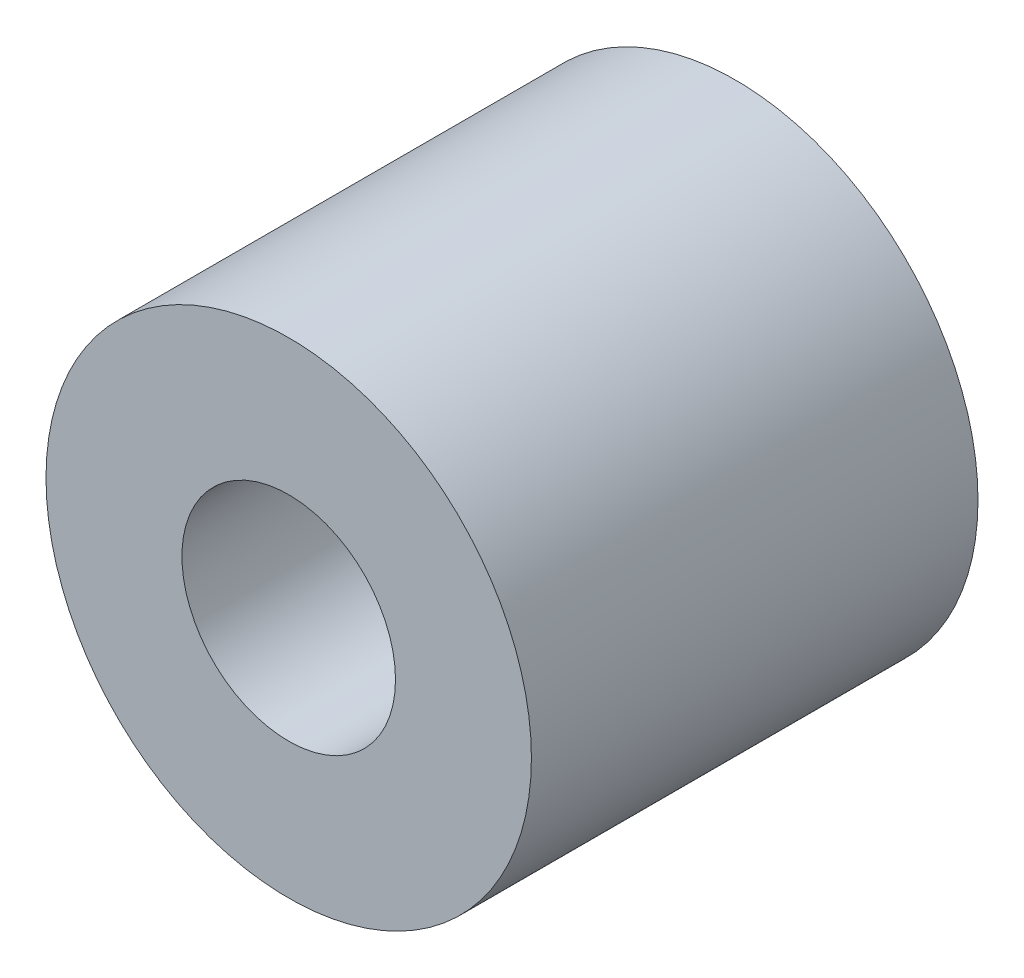
SolidWorks part; units mm, degrees
ref_plane "前视基准面" through (0, 0, 0) normal (0, 0, 1) x (1, 0, 0)
ref_plane "上视基准面" through (0, 0, 0) normal (0, 1, 0) x (1, 0, 0)
ref_plane "右视基准面" through (0, 0, 0) normal (1, 0, 0) x (0, 0, -1)
sketch "草图1" plane through (0, 0, 0) normal (0, 0, 1) x (1, 0, 0)
  circle A0 centre (0, 0) radius 12.5
  dimension "D1" = 25
extrude "凸台-拉伸1" add sketch "草图1" along normal blind 23
sketch "草图4" plane through (0, 0, 23) normal (0, 0, 1) x (1, 0, 0)
  point P0 (0, 0)
hole_wizard "M6 六角圆柱头螺钉的柱形沉头孔1" positions "草图4" profile "草图3" counterbore size "M6" standard "GB" end condition through all
sketch "草图3" plane through (0, 0, 23) normal (1, 0, 0) x (0, -1, 0)
  line L0 (0, 0) -> (0, 23)
  line L1 (0, 23) -> (3.3, 23)
  line L3 (3.3, 23) -> (3.3, 16.8)
  line L4 (3.3, 16.8) -> (5.5, 16.8)
  line L5 (5.5, 16.8) -> (5.5, 0)
  line L7 (5.5, 0) -> (0, 0)
  line L11 (0, -6.35) -> (0, 107.95) construction
  dimension "通孔孔直径" = 6.6
  dimension "通孔孔深度" = 23
  dimension "柱形沉头孔直径" = 11
  dimension "柱形沉头孔深度" = 16.8
